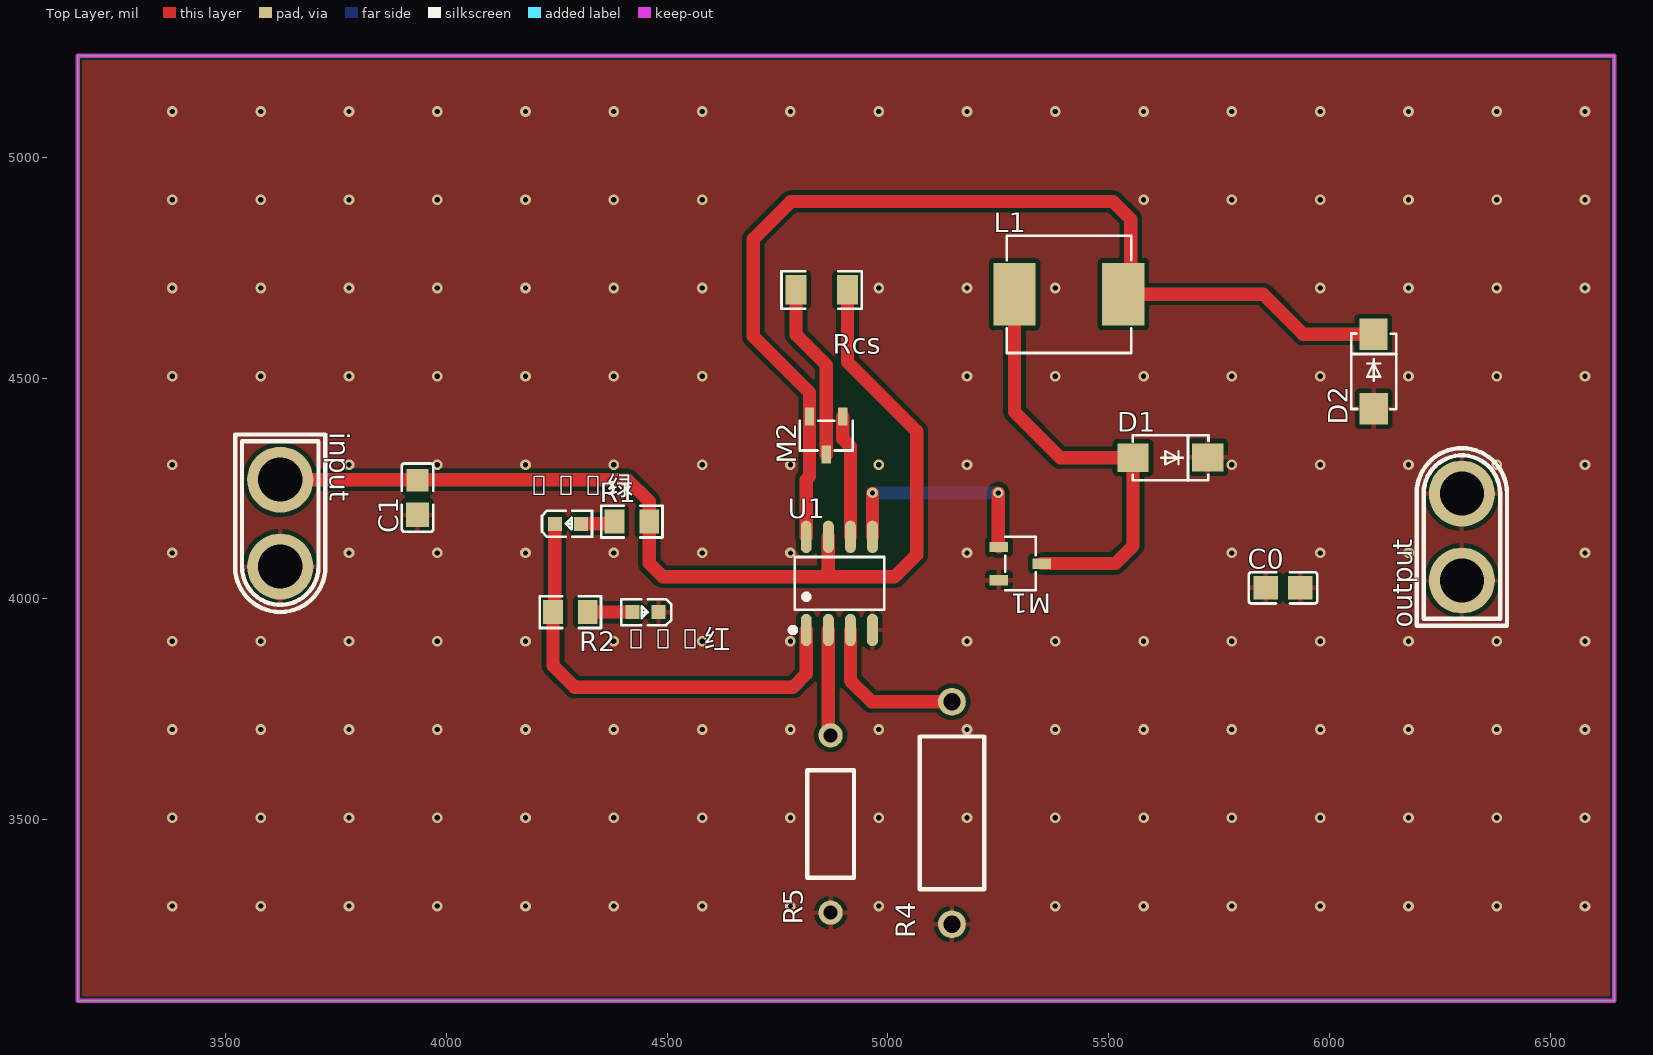
[diagram p0: Top Layer view]
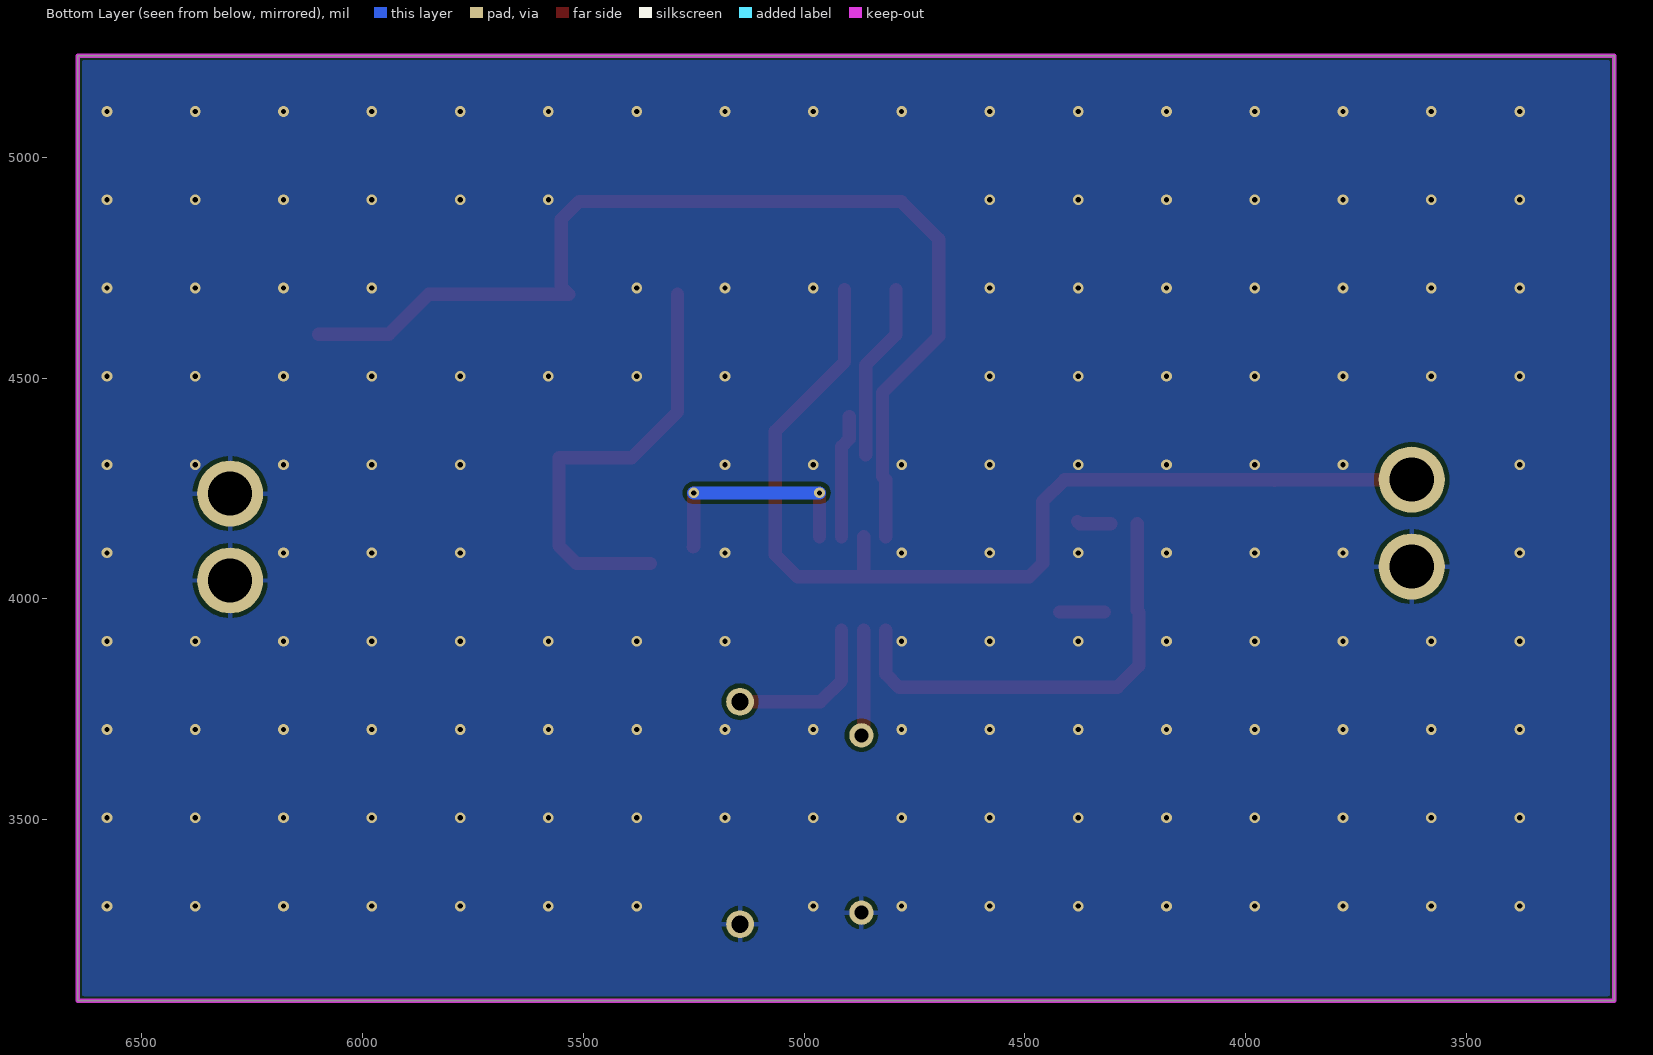
[diagram p1: Bottom Layer view, seen from below]
# Altium PCB MISC51207.pcbdoc
Units mil, origin at the board's own origin, x right, y up, seen from the top; angles counter-clockwise.
Board outline 3480 x 2140 mil, 2 copper layers (Top Layer, Bottom Layer), stack 62.206 mil thick; 17 components, 12 nets, 42 pads, 153 vias.

## Layer stack, top to bottom
Top Solder Mask Layer: solder mask 0.394, Dk 3.3
Top Layer: signal copper 1.379
Dielectric1: surface 59.449, FR4, Dk 4.5
Bottom Layer: signal copper 1.378
Bottom Solder Mask Layer: solder mask 0.394, Dk 3.3

## Board outline
3165,5230 3165,3090 6645,3090 6645,5230

## Design rules (kind name [scope] priority, off if disabled: settings)
BoardOutlineClearance copperThickness2oz_1 [All] p2 off: genericclearance=7.99 ignorepadtopadclearanceinfootprint=FALSE except(0: Arc-SplitContinuation Track-SplitContinuation SMDPad-SplitContinuation THPad-SplitContinuation Via-SplitContinuation Fill-SplitContinuation Region-SplitContinuation Poly-SplitContinuation Text-SplitContinuation Hole-SplitContinuation; 5.98: Arc-CutoutEdge SMDPad-CutoutEdge THPad-CutoutEdge Via-CutoutEdge Fill-CutoutEdge Region-CutoutEdge Text-CutoutEdge; 6.93: Hole-OutlineEdge Hole-CutoutEdge; 10: Poly-OutlineEdge Poly-CutoutEdge; 11.81: Arc-OutlineEdge Track-OutlineEdge SMDPad-OutlineEdge THPad-OutlineEdge Via-OutlineEdge Fill-OutlineEdge Region-OutlineEdge Text-OutlineEdge Track-CutoutEdge)
BoardOutlineClearance copperThickness1oz_1 [All] p4: genericclearance=4.02 ignorepadtopadclearanceinfootprint=FALSE except(0: Arc-SplitContinuation Track-SplitContinuation SMDPad-SplitContinuation THPad-SplitContinuation Via-SplitContinuation Fill-SplitContinuation Region-SplitContinuation Poly-SplitContinuation Text-SplitContinuation Hole-SplitContinuation; 6: SMDPad-CutoutEdge THPad-CutoutEdge Via-CutoutEdge Fill-CutoutEdge Region-CutoutEdge Text-CutoutEdge; 6.93: Hole-OutlineEdge Hole-CutoutEdge; 10: Poly-OutlineEdge Poly-CutoutEdge; 11.8: Arc-OutlineEdge Track-OutlineEdge SMDPad-OutlineEdge THPad-OutlineEdge Via-OutlineEdge Fill-OutlineEdge Region-OutlineEdge Text-OutlineEdge; 11.81: Arc-CutoutEdge Track-CutoutEdge)
Clearance copperThickness2oz [All] p1 off: gap=7.99 ignorepadtopadclearanceinfootprint=FALSE except(5.98: SMDPad-Track SMDPad-SMDPad THPad-Track SMDPad-THPad THPad-THPad Track-Via SMDPad-Via THPad-Via Via-Via Fill-Track Region-Track Fill-SMDPad Region-SMDPad Fill-THPad Region-THPad Fill-Via Region-Via Fill-Fill Fill-Region Region-Region Arc-Track Arc-SMDPad Arc-THPad Arc-Via Fill-Arc Region-Arc Arc-Arc Text-Track SMDPad-Text Text-THPad Text-Via Fill-Text Region-Text Arc-Text Text-Text; 6.93: Hole-Track Hole-SMDPad Hole-THPad Hole-Via Fill-Hole Region-Hole Hole-Arc Hole-Text; 10: Poly-Track Poly-SMDPad Poly-THPad Poly-Via Poly-Fill Poly-Region Poly-Poly Poly-Arc Poly-Text Poly-Hole)
Clearance copperThickness1oz [All] p3: gap=4.02 ignorepadtopadclearanceinfootprint=FALSE except(5.98: SMDPad-Track SMDPad-SMDPad THPad-Track SMDPad-THPad THPad-THPad Track-Via SMDPad-Via THPad-Via Via-Via Fill-Track Region-Track Fill-SMDPad Region-SMDPad Fill-THPad Region-THPad Fill-Via Region-Via Fill-Fill Fill-Region Region-Region; 6: Arc-Track Arc-SMDPad Arc-THPad Arc-Via Fill-Arc Region-Arc Arc-Arc Text-Track SMDPad-Text Text-THPad Text-Via Fill-Text Region-Text Arc-Text Text-Text; 6.93: Hole-Track Hole-SMDPad Hole-THPad Hole-Via Fill-Hole Region-Hole Hole-Arc Hole-Text; 10: Poly-Track Poly-SMDPad Poly-THPad Poly-Via Poly-Fill Poly-Region Poly-Poly Poly-Arc Poly-Text Poly-Hole)
DiffPairsRouting differentialPair [All] p1: maxlimit=6 minlimit=6 mostfreqgap=6 toplayer_minwidth=5 toplayer_prefwidth=10 toplayer_maxwidth=100 toplayer_mingap=6 toplayer_prefgap=6 toplayer_maxgap=6 bottomlayer_minwidth=5 bottomlayer_prefwidth=10 bottomlayer_maxwidth=100 bottomlayer_mingap=6 bottomlayer_prefgap=6 bottomlayer_maxgap=6 maxuncoupledlength=10
HoleToHoleClearance otherClearance [All] p1: gap=11.81 allowstackedmicrovias=TRUE
Length netLength [All] p1: minlimit=0 maxlimit=0
MatchedLengths netLengthTolerance [All] p1: tolerance=1000
PasteMaskExpansion pasteMaskExpansion [All] p1: expansion=0
PlaneConnect innerPlane [All] p1: planeconnectstyle=Relief reliefexpansion=20 reliefentries=4 reliefconductorwidth=10 reliefairgap=10
PolygonConnect copperRegion [(InNet('GND'))] p1: connectstyle=Relief reliefconductorwidth=10 reliefentries=4 polygonreliefangle="90 Angle" airgapwidth=10 via.connectstyle=Relief via.reliefconductorwidth=10 via.reliefentries=4 via.polygonreliefangle="90 Angle" via.airgapwidth=10
RoutingVias viaSize [All] p1: holewidth=12.01 width=24.02 viastyle="Through Hole" minholewidth=11.81 minwidth=19.68 maxholewidth=248.03 maxwidth=393.7
SolderMaskExpansion solderMaskExpansion [IsVia] p1: expansion=-1000 istentingtop=TRUE
SolderMaskExpansion solderMaskExpansion [All] p2: expansion=2 istentingtop=FALSE
Width copperThickness2oz_2 [All] p1 off: maxlimit=100 minlimit=8 preferedwidth=10
Width copperThickness1oz_2 [All] p2: maxlimit=100 minlimit=5 preferedwidth=10

## Components (designator, comment, footprint, x,y, rotation, side; value= is the part's Value field where it differs from the comment)
C0 "10uF" C0805#1 5895,4025 r0 top
C1 "10uF" C0805#2 3934.37,4229.37 r90 top
D1 "SS24" SMA_L4.3-W2.6-LS5.0-FD 5640,4320 r0 top
D2 "SS24" SMA_L4.3-W2.6-LS5.0-FD 6100,4515 r90 top
input "XT30U-M" CONN-TH_XT30U-M 3623.43,4171.57 r270 top
L1 "22uH" IND-SMD_L7.0-W6.6_FXL0630 5410,4690 r0 top
LED红 "NCD0603Y2" LED0603-RD 4450.74,3970 r180 top
LED绿 "NCD0603Y2" LED0603-RD 4275,4170 r0 top
M1 "SI2300DS-T1-GE3" SOT-23-3_L2.9-W1.6-P1.90-LS2.8-BR 5300,4080 r180 top
M2 "SI2301CDS-T1-GE3" SOT-23-3_L3.0-W1.7-P0.95-LS2.9-BR 4860,4370 r90 top
output "XT30U-M" CONN-TH_XT30U-M 6300,4140 r90 top
R1 "10kΩ" R0805 4420,4175 r0 top
R2 "10kΩ" R0805 4280.74,3970 r180 top
R4 "600kΩ" RES-TH_BD3.7-L8.7-P12.8-D0.8 5145,3515 r90 top
R5 "100kΩ" RES-TH_BD2.7-L6.2-P10.20-D0.4 4870,3490 r90 top
Rcs "150mΩ" R1206 4850,4700 r180 top
U1 "CN3305" SOP-8_L4.9-W3.9-P1.27-LS6.0-BL-1 4890,4035 r0 top

## Footprints (in the part's own frame and the unit in brackets; to place one, negate y for a bottom-side part, rotate by r counter-clockwise, add the part's x,y. Pads: shape width x height; smd on the part's side, far side on the other; paste and mask are expansions set on the pad)
C0805#1 [mm]
  rect 1.41x1.35 smd paste-100 mask+0.051: 1(-1,0) 2(1,0)
  silkscreen extent -1.96,-0.9 1.96,0.9
C0805#2 [mm]
  rect 1.41x1.35 smd paste-100 mask+0.051: 1(-1,0)
  rect 1.27x1.27 smd paste-100 mask+0.051: 2(1,0)
  silkscreen extent -1.96,-0.9 1.96,0.9
CONN-TH_XT30U-M [mm]
  round 3.8 hole 2.54 paste+0 mask+0.05: 1(-2.5,0) 2(2.5,0)
  silkscreen extent -5.1,-2.6 5.11,2.6
IND-SMD_L7.0-W6.6_FXL0630 [mm]
  rect 2.424x3.62 smd: 1(3.128,0) 2(-3.128,0)
  silkscreen extent -3.58,-3.38 3.58,3.38
LED0603-RD [mm]
  rect 0.8x0.8 smd: 1(-0.749,0) 2(0.749,0)
  silkscreen extent -1.49,-0.75 1.39,0.76
R0805 [mm]
  rect 1.133x1.377 smd paste-100 mask+0.051: 1(-1,0) 2(1,0)
  silkscreen extent -1.76,-0.92 1.76,0.92
R1206 [mil]
  rect 47.54x66.97 smd paste-3937.01 mask+2: 1(-58.22,0) 2(58.22,0)
  silkscreen extent -91,-42 91,42
RES-TH_BD2.7-L6.2-P10.20-D0.4 [mm]
  round 1.4 hole 0.8 copper offset 0,0: 1(-5.1,0) 2(5.1,0)
  silkscreen extent -3.1,-1.35 3.1,1.35
RES-TH_BD3.7-L8.7-P12.8-D0.8 [mm]
  round 1.6 hole 1: 1(-6.4,0) 2(6.4,0)
  silkscreen extent -4.4,-1.85 4.4,1.85
SMA_L4.3-W2.6-LS5.0-FD [mm]
  rect 1.8x1.62 smd: 1(-2.15,-0.009) 2(2.15,0.009)
  silkscreen extent -2.17,-1.32 2.19,1.29
SOP-8_L4.9-W3.9-P1.27-LS6.0-BL-1 [mm]
  oval 0.63x1.865 smd: 1(-1.905,-2.683) 2(-0.635,-2.683) 3(0.635,-2.683) 4(1.905,-2.683) 5(1.905,2.682) 6(0.635,2.682) 7(-0.635,2.682) 8(-1.905,2.682)
  silkscreen extent -2.82,-2.83 2.58,1.52
SOT-23-3_L2.9-W1.6-P1.90-LS2.8-BR [mm]
  rect 1.07x0.6 smd: 1(1.235,-0.95) 2(1.235,0.95) 3(-1.235,0)
  silkscreen extent -0.88,-1.54 0.88,1.54
SOT-23-3_L3.0-W1.7-P0.95-LS2.9-BR [mil]
  rect 40.85x20.95 smd: 1(43.36,-37.4) 2(43.36,37.4) 3(-43.36,0)
  silkscreen extent -34,-60 34,60

## Via types
v1: diameter 24.02, hole 12, Top Layer to Bottom Layer, 153 vias

## Nets (pads, with @x,y where several pads share a name; then routed paths per layer and width w, separated by ;. In a path a pad name is that pad's centre, name@x,y a point inside that pad or via, vN(x,y) a via of type N, cw(c..) or ccw(c..) an arc to the next point about the centre after c; other vN are vias at no path point)
$1N1: C1.2 input.1 R1.2 Rcs.1 U1.7 | length 2392.8
  Top Layer w30: input.1 C1.2@3933.11,4270 ; C1.2 C1.2@3933.11,4270 ; U1.7 4865,4050 ; Rcs.1 4908.22,4536.78 5065,4380 5065,4100 5015,4050 4865,4050 ; C1.2@3933.11,4270 4410,4270 4459.37,4220.63 R1.2 4459.37,4080.63 4490,4050 4865,4050
$1N6: M1.1 U1.5 | length 507.6
  Top Layer w30: U1.5 v1(4965,4240) ; v1(5250,4240) 5250,4118.77 M1.1
  Bottom Layer w30: v1(4965,4240) v1(5250,4240)
$1N9: R5.2 U1.2 | length 240.7
  Top Layer w30: U1.2 4865,3695.79 R5.2
$1N10: R4.2 U1.3 | length 364.3
  Top Layer w30: U1.3 4915,3815 4963.03,3766.97 R4.2
$1N11: M2.3 Rcs.2 | length 401.6
  Top Layer w30: Rcs.2 4791.78,4598.22 4860,4530 M2.3
$1N17: D2.2 L1.1 M2.2 U1.8 | length 2418.1
  Top Layer w30: U1.8 4815,4270 4822.6,4277.6 M2.2 4822.6,4467.4 4695,4595 4695,4815 4780,4900 5510,4900 5550,4860 5550,4706.85 L1.1 5850,4690 5940.35,4599.65 D2.2
$1N18: M2.1 U1.6 | length 280
  Top Layer w30: M2.1 4897.4,4362.6 4915,4345 U1.6
$1N19: LED绿.2 R1.1 | length 78.2
  Top Layer w30: LED绿.2 4375.64,4170.01 R1.1
$1N20: LED红.2 R2.1 | length 101.1
  Top Layer w30: R2.1 LED红.2
$1N21: D1.1 L1.2 M1.3 | length 1001
  Top Layer w30: L1.2 5286.85,4423.15 5390.37,4319.63 D1.1 5555.35,4120.35 5515,4080 M1.3
$1N25: LED绿.1 R2.2 U1.1 | length 1028.7
  Top Layer w30: LED绿.1 4245.51,3974.14 R2.2 4241.37,3848.63 4290,3800 4785,3800 4815,3830 U1.1
GND: C0.1 C0.2 C1.1 D1.2 D2.1 input.2 LED红.1 M1.2 output.1 output.2 R4.1 R5.1 U1.4
  other v1: 3379.1,3304.1 3579.1,3304.1 3779.1,3304.1 3979.1,3304.1 4179.1,3304.1 4379.1,3304.1 4579.1,3304.1 4779.1,3304.1 4979.1,3304.1 5379.1,3304.1 5579.1,3304.1 5779.1,3304.1 5979.1,3304.1 6179.1,3304.1 6379.1,3304.1 6579.1,3304.1 3379.1,3504.1 3579.1,3504.1 3779.1,3504.1 3979.1,3504.1 4179.1,3504.1 4379.1,3504.1 4579.1,3504.1 4779.1,3504.1 4979.1,3504.1 5179.1,3504.1 5379.1,3504.1 5579.1,3504.1 5779.1,3504.1 5979.1,3504.1 6179.1,3504.1 6379.1,3504.1 6579.1,3504.1 3379.1,3704.1 3579.1,3704.1 3779.1,3704.1 3979.1,3704.1 4179.1,3704.1 4379.1,3704.1 4579.1,3704.1 4779.1,3704.1 4979.1,3704.1 5179.1,3704.1 5379.1,3704.1 5579.1,3704.1 5779.1,3704.1 5979.1,3704.1 6179.1,3704.1 6379.1,3704.1 6579.1,3704.1 3379.1,3904.1 3579.1,3904.1 3779.1,3904.1 3979.1,3904.1 4179.1,3904.1 4379.1,3904.1 4579.1,3904.1 4779.1,3904.1 5179.1,3904.1 5379.1,3904.1 5579.1,3904.1 5779.1,3904.1 5979.1,3904.1 6179.1,3904.1 6379.1,3904.1 6579.1,3904.1 3379.1,4104.1 3779.1,4104.1 3979.1,4104.1 4179.1,4104.1 4379.1,4104.1 4579.1,4104.1 4779.1,4104.1 5179.1,4104.1 5779.1,4104.1 5979.1,4104.1 6179.1,4104.1 6579.1,4104.1 3379.1,4304.1 3779.1,4304.1 3979.1,4304.1 4179.1,4304.1 4379.1,4304.1 4579.1,4304.1 4779.1,4304.1 4979.1,4304.1 5179.1,4304.1 5779.1,4304.1 5979.1,4304.1 6179.1,4304.1 6379.1,4304.1 6579.1,4304.1 3379.1,4504.1 3579.1,4504.1 3779.1,4504.1 3979.1,4504.1 4179.1,4504.1 4379.1,4504.1 4579.1,4504.1 5179.1,4504.1 5379.1,4504.1 5579.1,4504.1 5779.1,4504.1 5979.1,4504.1 6179.1,4504.1 6379.1,4504.1 6579.1,4504.1 3379.1,4704.1 3579.1,4704.1 3779.1,4704.1 3979.1,4704.1 4179.1,4704.1 4379.1,4704.1 4579.1,4704.1 4979.1,4704.1 5179.1,4704.1 5379.1,4704.1 5979.1,4704.1 6179.1,4704.1 6379.1,4704.1 6579.1,4704.1 3379.1,4904.1 3579.1,4904.1 3779.1,4904.1 3979.1,4904.1 4179.1,4904.1 4379.1,4904.1 4579.1,4904.1 5579.1,4904.1 5779.1,4904.1 5979.1,4904.1 6179.1,4904.1 6379.1,4904.1 6579.1,4904.1 3379.1,5104.1 3579.1,5104.1 3779.1,5104.1 3979.1,5104.1 4179.1,5104.1 4379.1,5104.1 4579.1,5104.1 4779.1,5104.1 4979.1,5104.1 5179.1,5104.1 5379.1,5104.1 5579.1,5104.1 5779.1,5104.1 5979.1,5104.1 6179.1,5104.1 6379.1,5104.1 6579.1,5104.1

## Polygon pours and split planes (outlines as drawn)
GND on Top Layer (solid, remove dead copper, pour order 0): 3065,5480 3065,3075 6920,3075 6920,5480
GND on Bottom Layer (solid, remove dead copper, pour order 2): 3000,5435 3000,3000 6850,3000 6850,5435

## Keep-outs
Board Outline Layer:
  the board outline again, w10